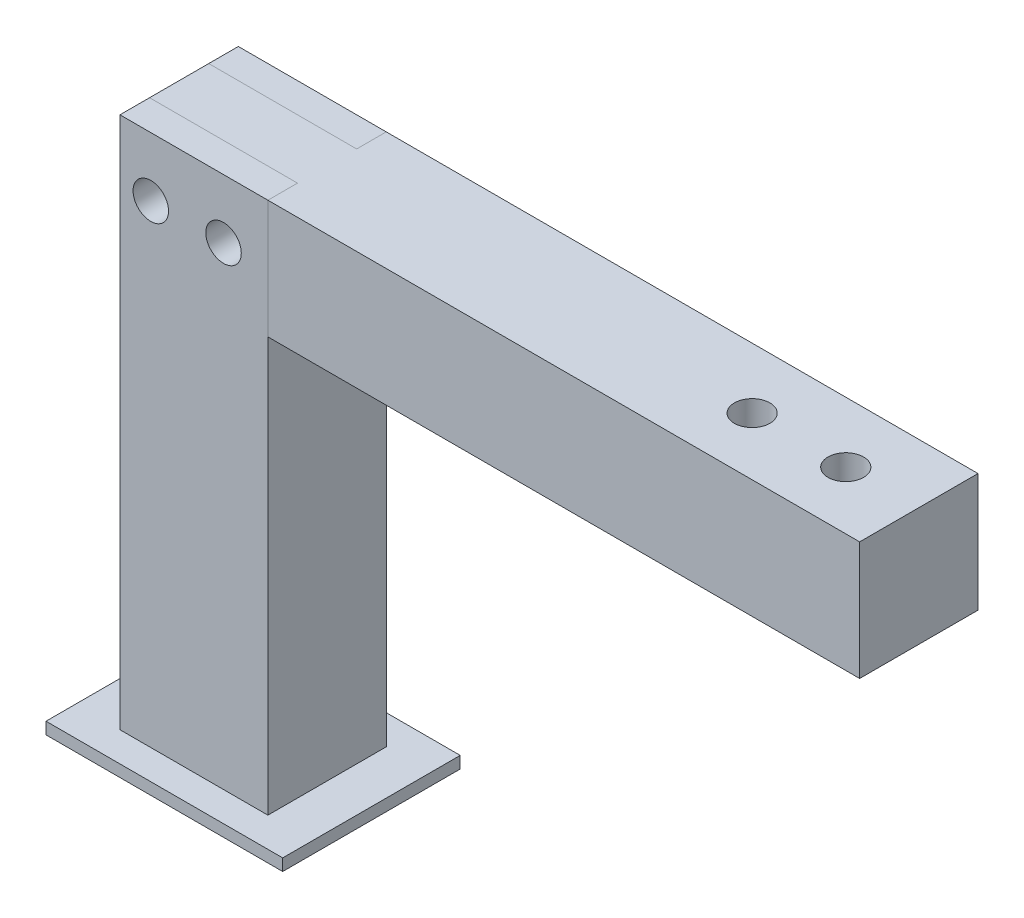
from build123d import *

# Parameters (mm, degrees)
SKETCH1_W           = 40
SKETCH1_H           = 30
BOSS_EXTRUDE1_DEPTH = 2
SKETCH5_W           = 25
SKETCH5_H           = 20
BOSS_EXTRUDE2_DEPTH = 90
SKETCH6_W           = 25
SKETCH6_H           = 10
CUT_EXTRUDE3_DEPTH  = 20
BOSS_EXTRUDE3_DEPTH = 20
SKETCH8_R           = 3
CUT_EXTRUDE4_DEPTH  = 20
SKETCH9_R           = 3
CUT_EXTRUDE5_DEPTH  = 29


with BuildPart() as part:
    # Sketch1 → Boss-Extrude1 (new body)
    with BuildSketch(Plane(origin=(0, 0, 0), x_dir=(1, 0, 0), z_dir=(0, 1, 0))):
        with Locations((-5, 0.243631658)):
            Rectangle(SKETCH1_W, SKETCH1_H)
    extrude(amount=BOSS_EXTRUDE1_DEPTH)

    # Sketch5 → Boss-Extrude2 (add)
    with BuildSketch(Plane(origin=(0, 2, 0), x_dir=(1, 0, 0), z_dir=(0, 1, 0))):
        with Locations((-5, 0.243631658)):
            Rectangle(SKETCH5_W, SKETCH5_H)
    extrude(amount=BOSS_EXTRUDE2_DEPTH)

    # Sketch6 → Cut-Extrude3 (cut)
    with BuildSketch(Plane(origin=(0, 92, 0), x_dir=(1, 0, 0), z_dir=(0, 1, 0))):
        with Locations((-5, 0.243631658)):
            Rectangle(SKETCH6_W, SKETCH6_H)
    extrude(amount=-CUT_EXTRUDE3_DEPTH, mode=Mode.SUBTRACT)


with BuildPart() as body_2:
    # Sketch7 → Boss-Extrude3 (new body)
    with BuildSketch(Plane(origin=(0, 72, 0), x_dir=(1, 0, 0), z_dir=(0, 1, 0))):
        Polygon((7.5, -4.756368342), (7.5, -9.756368342), (107.5, -9.756368342), (107.5, 10.243631658), (7.5, 10.243631658), (7.5, 5.243631658), (-17.5, 5.243631658), (-17.5, -4.756368342), align=None)
    extrude(amount=BOSS_EXTRUDE3_DEPTH)

    # Sketch8 → Cut-Extrude4 (cut)
    with BuildSketch(Plane(origin=(0, 92, 0), x_dir=(1, 0, 0), z_dir=(0, 1, 0))):
        with Locations(Location((95.398148597, 0, 0), (0, 0, 270))):
            Circle(SKETCH8_R)
        with Locations(Location((79.574536826, 0, 0), (0, 0, 270))):
            Circle(SKETCH8_R)
    extrude(amount=-CUT_EXTRUDE4_DEPTH, mode=Mode.SUBTRACT)


with BuildPart() as cut_extrude5_tool:
    # Sketch9 → Cut-Extrude5 (new body)
    with BuildSketch(Plane.XY.offset(9.756368342)):
        with Locations((-12.290030702, 82)):
            Circle(SKETCH9_R)
        with Locations((0, 82)):
            Circle(SKETCH9_R)
    extrude(amount=-CUT_EXTRUDE5_DEPTH)


with BuildPart() as part_1:
    add(part.part)

    # Cut-Extrude5: cut by cut_extrude5_tool
    add(cut_extrude5_tool.part, mode=Mode.SUBTRACT)


with BuildPart() as body_2_1:
    add(body_2.part)

    # Cut-Extrude5: cut by cut_extrude5_tool
    add(cut_extrude5_tool.part, mode=Mode.SUBTRACT)


solid = Compound([part_1.part, body_2_1.part])
